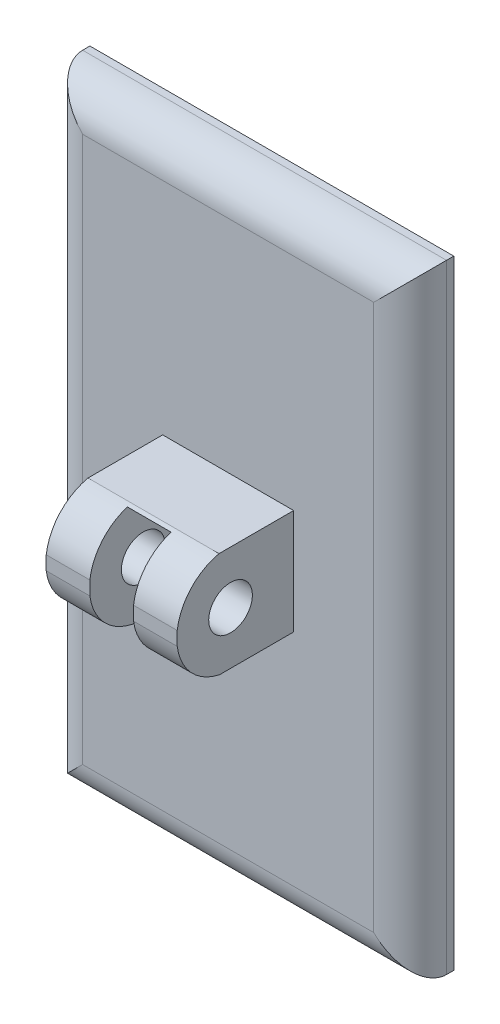
from build123d import *

# Parameters (mm, degrees)
SKETCH1_W           = 50
SKETCH1_H           = 85
BOSS_EXTRUDE1_DEPTH = 6
SKETCH2_W           = 18
SKETCH2_H           = 14.448315912
BOSS_EXTRUDE2_DEPTH = 16
FILLET1_R           = 5
SKETCH3_W           = 6
SKETCH3_H           = 29.716496746
CUT_EXTRUDE1_DEPTH  = 16
SKETCH4_R           = 3
CUT_EXTRUDE2_DEPTH  = 95.154128959


with BuildPart() as part:
    # Sketch1 → Boss-Extrude1 (new body)
    with BuildSketch(Plane.XY):
        with Locations((25, 42.5)):
            Rectangle(SKETCH1_W, SKETCH1_H)
    extrude(amount=BOSS_EXTRUDE1_DEPTH)

    # Sketch2 → Boss-Extrude2 (add)
    with BuildSketch(Plane.XY.offset(6)):
        with Locations((25, 42.5)):
            Rectangle(SKETCH2_W, SKETCH2_H)
    extrude(amount=BOSS_EXTRUDE2_DEPTH)

    # Fillet1
    fillet1_edges = [part.edges().sort_by_distance(p)[0] for p in [
        (50, 42.5, 6),
        (25, 85, 6),
        (0, 42.5, 6),
        (25, 0, 6),
    ]]
    fillet(fillet1_edges, radius=FILLET1_R)

    # Sketch3 → Cut-Extrude1 (cut)
    with BuildSketch(Plane.XY.offset(22)):
        with Locations((25, 34.711959109)):
            Rectangle(SKETCH3_W, SKETCH3_H)
    extrude(amount=-CUT_EXTRUDE1_DEPTH, mode=Mode.SUBTRACT)

    # Sketch4 → Cut-Extrude2 (cut, through all)
    with BuildSketch(Plane.ZY.offset(-16)):
        with Locations(Location((14.673320443, 42.507843144, 0), (0, 0, 270))):
            Circle(SKETCH4_R)
        with BuildLine():
            Line((14.673320443, 49.895764166), (20.802104858, 55.115800091))
            Line((20.802104858, 55.115800091), (35.798114719, 48.402784846))
            Line((35.798114719, 48.402784846), (20.212830652, 12.710723094))
            Line((20.212830652, 12.710723094), (14.673320443, 35.119922122))
            ThreePointArc((14.673320443, 35.119922122), (22.061241465, 42.507843144), (14.673320443, 49.895764166))
        make_face()
    extrude(amount=-CUT_EXTRUDE2_DEPTH, mode=Mode.SUBTRACT)


solid = part.part
